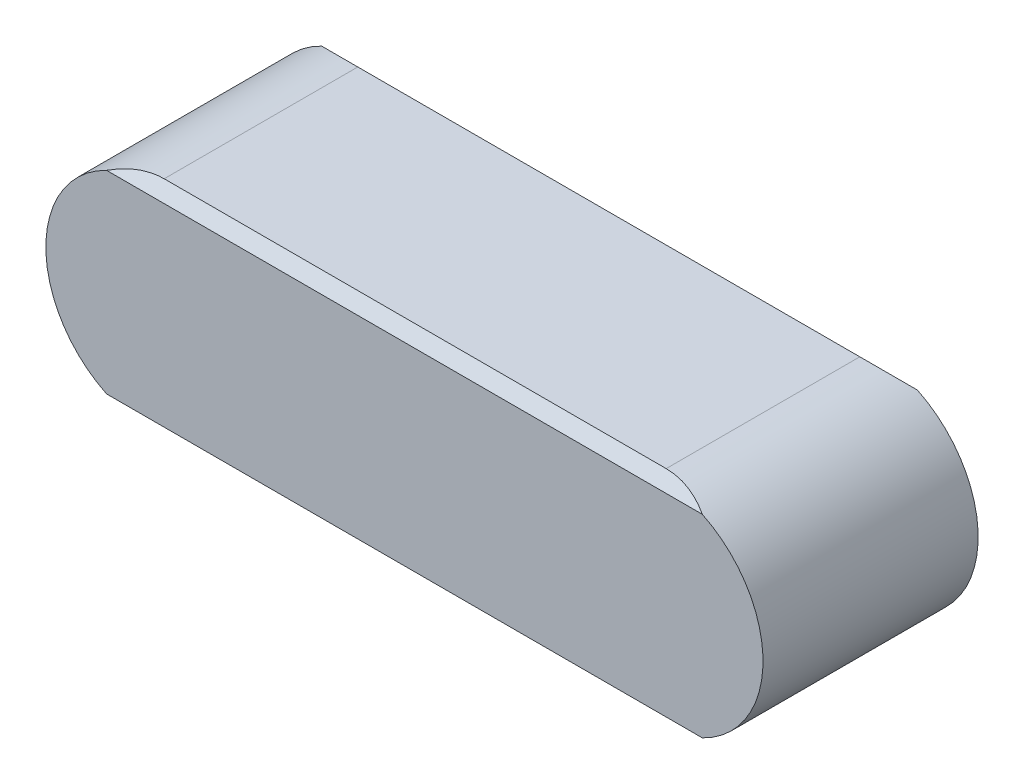
SolidWorks part; units mm, degrees
material "SUS304"
ref_plane "前视基准面" through (0, 0, 0) normal (0, 0, 1) x (1, 0, 0)
ref_plane "上视基准面" through (0, 0, 0) normal (0, 1, 0) x (1, 0, 0)
ref_plane "右视基准面" through (0, 0, 0) normal (1, 0, 0) x (0, 0, -1)
ref_plane "基准面1" through (0, 0, 0) normal (0, 0, 1) x (1, 0, 0)
sketch "草图1" plane through (0, 0, 0) normal (0, 0, 1) x (1, 0, 0)
  line L0 (3, 0) -> (17, 0)
  line L1 (17, 6) -> (3, 6)
  arc A0 (0, 3) -> (3, 0) centre (3, 3) ccw
  arc A1 (17, 0) -> (20, 3) centre (17, 3) ccw
  arc A2 (20, 3) -> (17, 6) centre (17, 3) ccw
  arc A3 (3, 6) -> (0, 3) centre (3, 3) ccw
extrude "凸台-拉伸1" add sketch "草图1" along normal blind 6
ref_plane "基准面2" through (0, 0, 0) normal (1, 0, 0) x (0, 0, -1)
sketch "草图2" plane through (0, 0, 0) normal (1, 0, 0) x (0, 0, -1)
  line L0 (-9, -3) -> (3, -3)
  line L1 (3, -3) -> (3, 9)
  line L2 (3, 9) -> (-9, 9)
  line L3 (-9, 9) -> (-9, -3)
  line L4 (-6, 5.7) -> (-6, 0.3)
  line L5 (-6, 0.3) -> (-5.7, 0)
  line L6 (-5.7, 0) -> (-0.3, 0)
  line L7 (-0.3, 0) -> (0, 0.3)
  line L8 (0, 0.3) -> (0, 5.7)
  line L9 (0, 5.7) -> (-0.3, 6)
  line L10 (-0.3, 6) -> (-5.7, 6)
  line L11 (-5.7, 6) -> (-6, 5.7)
extrude "切除-拉伸1" cut sketch "草图2" along normal blind 20
